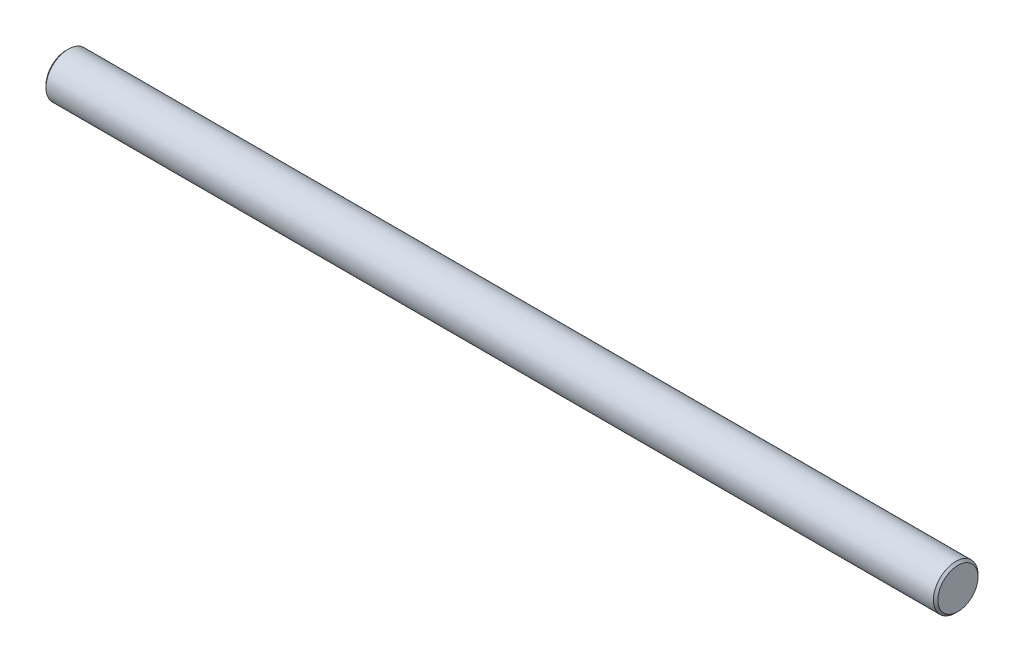
from build123d import *

# Parameters (mm, degrees)
SKETCH_1_R           = 1.5
EXTRUDE_1_DEPTH      = 30
CHAMFER_C0_15_1_SIZE = 0.15


with BuildPart() as part:
    # 草图1 → 凸台-拉伸1 (new, symmetric)
    with BuildSketch(Plane(origin=(0, 0, 0), x_dir=(0, 0, -1), z_dir=(1, 0, 0))):
        Circle(SKETCH_1_R)
    extrude(amount=EXTRUDE_1_DEPTH, both=True)

    # C0.15 倒角1
    chamfer_c0_15_1_edges = [part.edges().sort_by_distance(p)[0] for p in [
        (-30, 0, 1.5),
        (30, 0, 1.5),
    ]]
    chamfer(chamfer_c0_15_1_edges, length=CHAMFER_C0_15_1_SIZE)


solid = part.part
